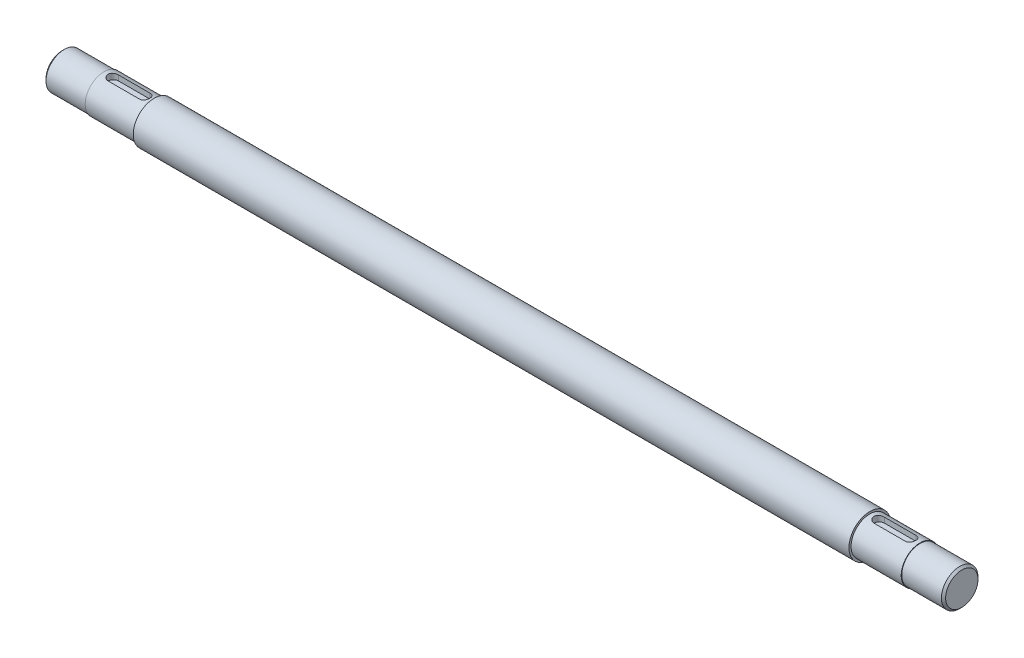
from build123d import *

# Parameters (mm, degrees)
SKETCH_1_R          = 20
EXTRUDE_1_DEPTH     = 342.5
SKETCH_2_R          = 18
EXTRUDE_2_DEPTH     = 48
SKETCH_3_R          = 17.5
EXTRUDE_3_DEPTH     = 40
EXTRUDE_START       = 48
SKETCH_4_R          = 18
EXTRUDE_4_DEPTH     = 48
EXTRUDE_START_2     = 40
SKETCH_5_R          = 17.5
EXTRUDE_5_DEPTH     = 40
CUT_EXTRUDE_1_DEPTH = 5.71
CHAMFER_1_SIZE      = 2


with BuildPart() as part:
    # 草图1 → 凸台-拉伸1 (new, symmetric)
    with BuildSketch(Plane(origin=(0, 0, 0), x_dir=(0, 0, -1), z_dir=(1, 0, 0))):
        Circle(SKETCH_1_R)
    extrude(amount=EXTRUDE_1_DEPTH, both=True)

    # 草图2 → 凸台-拉伸2 (add)
    with BuildSketch(Plane.ZY.offset(342.5)):
        with Locations(Location((0, 0, 0), (0, 0, 180))):
            Circle(SKETCH_2_R)
    extrude(amount=EXTRUDE_2_DEPTH)

    # 草图3 → 凸台-拉伸3 (add)
    with BuildSketch(Plane.ZY.offset(390.5)):
        Circle(SKETCH_3_R)
    extrude(amount=EXTRUDE_3_DEPTH)

    # 草图4 → 凸台-拉伸4 (add)
    with BuildSketch(Plane(origin=(342.5, 0, 0), x_dir=(0, 0, -1), z_dir=(1, 0, 0)).offset(EXTRUDE_START)):
        Circle(SKETCH_4_R)
    extrude(amount=-EXTRUDE_4_DEPTH)

    # 草图5 → 凸台-拉伸5 (add)
    with BuildSketch(Plane(origin=(390.5, 0, 0), x_dir=(0, 0, -1), z_dir=(1, 0, 0)).offset(EXTRUDE_START_2)):
        with Locations(Location((0, 0, 0), (0, 0, 180))):
            Circle(SKETCH_5_R)
    extrude(amount=-EXTRUDE_5_DEPTH)

    # 草图7 → 切除-拉伸1 (cut)
    with BuildSketch(Plane(origin=(0, 18, 0), x_dir=(1, 0, 0), z_dir=(0, 1, 0))):
        with BuildLine():
            Line((351.5, 5), (381.5, 5))
            ThreePointArc((381.5, 5), (386.5, 0), (381.5, -5))
            Line((381.5, -5), (351.5, -5))
            ThreePointArc((351.5, -5), (346.5, 0), (351.5, 5))
        make_face()
        with BuildLine():
            Line((-351.5, -5), (-381.5, -5))
            ThreePointArc((-381.5, -5), (-386.5, 0), (-381.5, 5))
            Line((-381.5, 5), (-351.5, 5))
            ThreePointArc((-351.5, 5), (-346.5, 0), (-351.5, -5))
        make_face()
    extrude(amount=-CUT_EXTRUDE_1_DEPTH, mode=Mode.SUBTRACT)

    # 倒角1
    chamfer_1_edges = [part.edges().sort_by_distance(p)[0] for p in [
        (-430.5, 0, -17.5),
        (430.5, 0, -17.5),
    ]]
    chamfer(chamfer_1_edges, length=CHAMFER_1_SIZE)


solid = part.part
